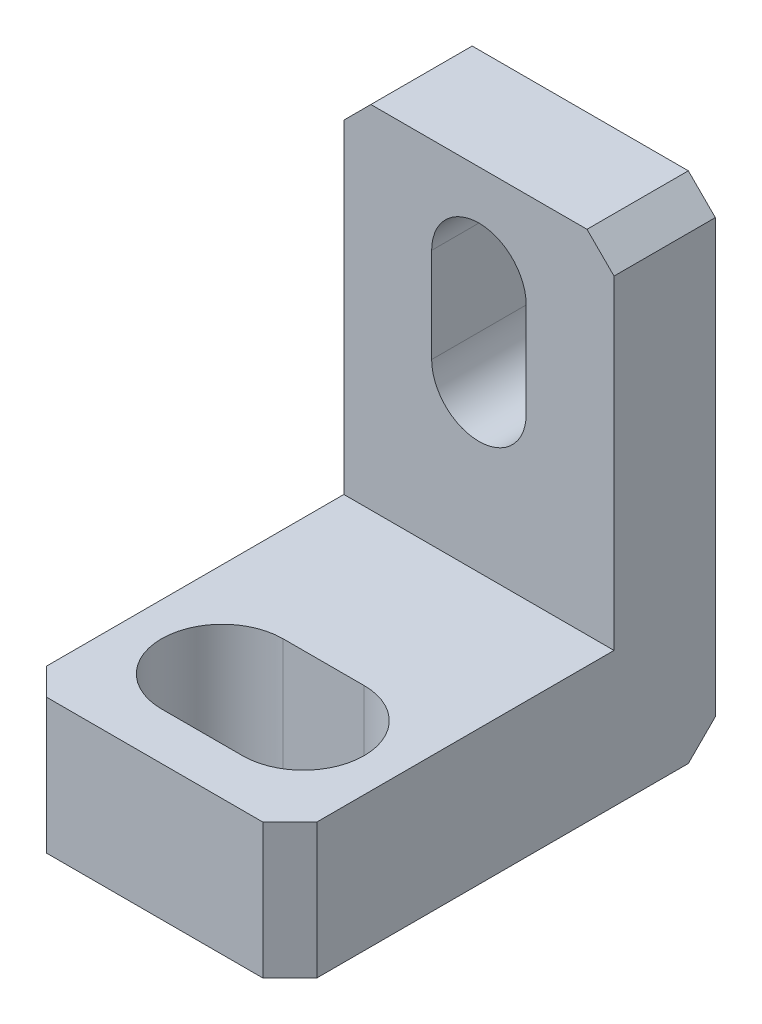
SolidWorks part; units mm, degrees
ref_plane "Front Plane" through (0, 0, 0) normal (0, 0, 1) x (1, 0, 0)
ref_plane "Top Plane" through (0, 0, 0) normal (0, 1, 0) x (1, 0, 0)
ref_plane "Right Plane" through (0, 0, 0) normal (1, 0, 0) x (0, 0, -1)
sketch "Sketch1" plane through (0, 0, 0) normal (0, 1, 0) x (1, 0, 0)
  line L1 (0, 0) -> (10, 0)
  line L2 (0, 0) -> (0, 3.75)
  line L3 (0, 3.75) -> (10, 3.75)
  line L4 (10, 0) -> (10, 3.75)
  dimension "D1" = 10
extrude "Boss-Extrude1" add sketch "Sketch1" along normal blind 18
sketch "Sketch2" plane through (0, 0, 0) normal (0, 0, 1) x (1, 0, 0)
  line L0 (5, 18) -> (5, 0) construction
  line L1 (0, 18) -> (10, 18) construction
  line L2 (0, 0) -> (10, 0) construction
  circle A0 centre (5, 12.7) radius 1.75
  dimension "D1" = 12.7
  dimension "D2" = 3.5
extrude "Cut-Extrude1" cut sketch "Sketch2" against normal blind 20
sketch "Sketch3" plane through (0, 0, 0) normal (0, -1, 0) x (1, 0, 0)
  line L1 (0, 0) -> (10, 0)
  line L2 (0, 0) -> (0, 12)
  line L3 (0, 12) -> (10, 12)
  line L4 (10, 0) -> (10, 12)
  dimension "D2" = 12
extrude "Boss-Extrude2" add sketch "Sketch3" against normal blind 5
sketch "Sketch4" plane through (0, 5, 0) normal (0, 1, 0) x (1, 0, 0)
  line L2 (5, -12) -> (5, -4.5861) construction
  line L4 (3.5, -10.25) -> (6.5, -10.25)
  line L5 (3.5, -5.75) -> (6.5, -5.75)
  line L10 (10, -12) -> (0, -12) construction
  arc A0 (3.5, -5.75) -> (3.5, -10.25) centre (3.5, -8) ccw
  arc A1 (6.5, -10.25) -> (6.5, -5.75) centre (6.5, -8) ccw
  dimension "D1" = 4
  dimension "D2" = 3
  dimension "D3" = 4.5
extrude "Cut-Extrude2" cut sketch "Sketch4" against normal blind 10
chamfer "Chamfer1" distance 1 angle 45 5 edges at (0, 2.5, 12) (10, 2.5, 12) (10, 18, -1.875) (0, 18, -1.875) (5, 0, -3.75)
sketch "Sketch5" plane through (0, 0, 0) normal (0, 0, 1) x (1, 0, 0)
  line L0 (5, 14.45) -> (5, 10.95) construction
  line L1 (6.75, 14.45) -> (6.75, 10.95)
  line L2 (3.25, 14.45) -> (3.25, 10.95)
  arc A0 (6.75, 14.45) -> (3.25, 14.45) centre (5, 14.45) ccw
  arc A1 (3.25, 10.95) -> (6.75, 10.95) centre (5, 10.95) ccw
  circle A2 centre (5, 12.7) radius 1.75 construction
  point P2 (5, 12.7)
  dimension "D1" = 3.5
extrude "Cut-Extrude3" cut sketch "Sketch5" against normal blind 10
